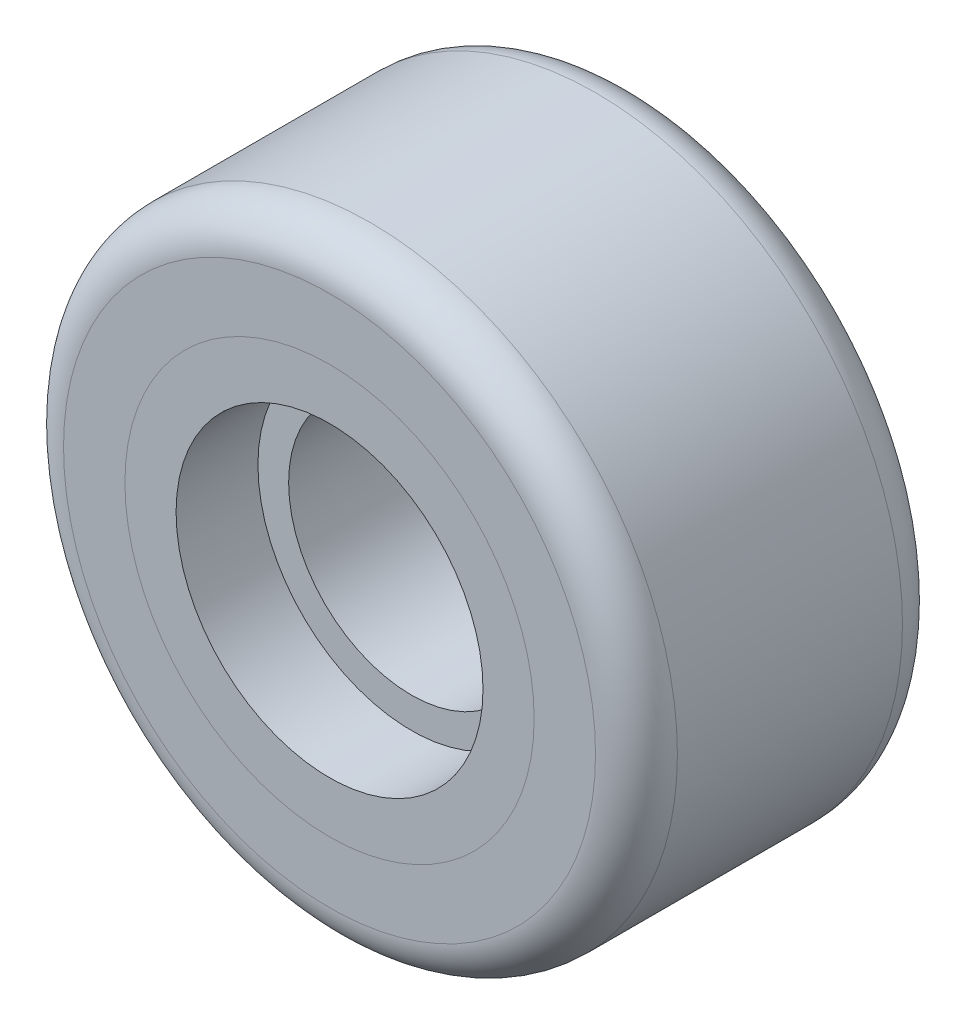
SolidWorks part; units mm, degrees
material "A6061+优力胶"
ref_plane "Front Plane" through (0, 0, 0) normal (0, 0, 1) x (1, 0, 0)
ref_plane "Top Plane" through (0, 0, 0) normal (0, 1, 0) x (1, 0, 0)
ref_plane "Right Plane" through (0, 0, 0) normal (1, 0, 0) x (0, 0, -1)
sketch "Sketch1" plane through (0, 0, 0) normal (0, 0, 1) x (1, 0, 0)
  circle A0 centre (0, 0) radius 10
  dimension "D1" = 20
extrude "Boss-Extrude1" add sketch "Sketch1" along normal blind 15
sketch "Sketch2" plane through (0, 0, 15) normal (0, 0, 1) x (1, 0, 0)
  circle A0 centre (0, 0) radius 15
  circle A1 centre (0, 0) radius 10
  dimension "D1" = 30
  dimension "D2" = 20
extrude "Boss-Extrude2" add sketch "Sketch2" against normal up to surface (15 mm away) separate body up to face at (10, 0, 0)
sketch "Sketch3" plane through (0, 0, 15) normal (0, 0, 1) x (1, 0, 0)
  circle A0 centre (0, 0) radius 6
  dimension "D1" = 12
extrude "Cut-Extrude1" cut sketch "Sketch3" against normal through all
sketch "Sketch4" plane through (0, 0, 15) normal (0, 0, 1) x (1, 0, 0)
  circle A0 centre (0, 0) radius 7.5
  dimension "D1" = 15
extrude "Cut-Extrude2" cut sketch "Sketch4" against normal blind 4
sketch "Sketch5" plane through (0, 0, 0) normal (0, 0, -1) x (-1, 0, 0)
  circle A0 centre (0, 0) radius 7.5
  dimension "D1" = 15
extrude "Cut-Extrude3" cut sketch "Sketch5" against normal blind 4
fillet "Fillet1" radius 2 2 edges at (15, 0, 0) (15, 0, 15)
